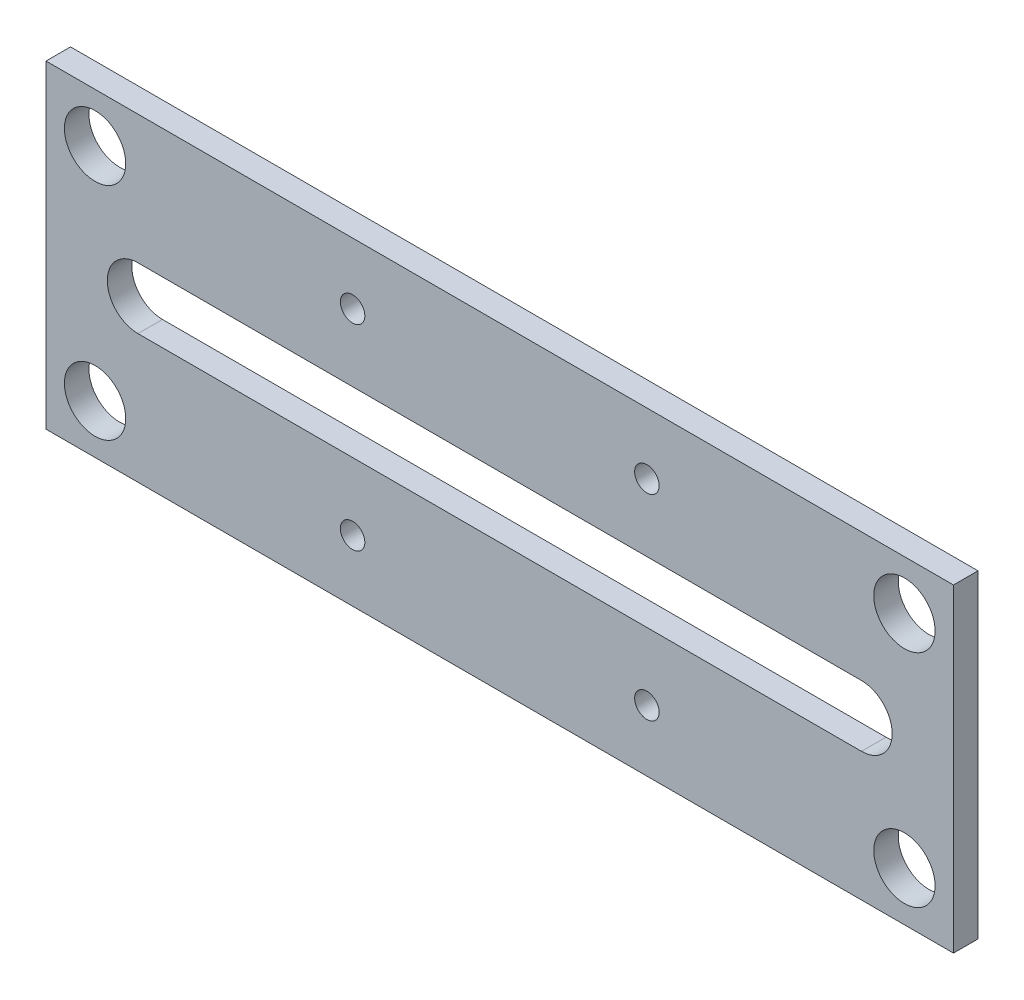
SolidWorks part; units mm, degrees
ref_plane "Front Plane" through (0, 0, 0) normal (0, 0, 1) x (1, 0, 0)
ref_plane "Top Plane" through (0, 0, 0) normal (0, 1, 0) x (1, 0, 0)
ref_plane "Right Plane" through (0, 0, 0) normal (1, 0, 0) x (0, 0, -1)
ref_plane "Plane1" through (0, 0, 0) normal (0, 0, -1) x (-1, 0, 0)
sketch "Sketch1" plane through (0, 0, 0) normal (0, 0, -1) x (-1, 0, 0)
  line L0 (-185, 0) -> (-185, 6.1768) construction
  line L1 (0, 0) -> (0, 130)
  line L3 (0, 130) -> (-370, 130)
  line L5 (-370, 130) -> (-370, 0)
  line L7 (-370, 0) -> (0, 0)
  line L8 (-37.5, 52.5) -> (-332.5, 52.5)
  line L9 (-332.5, 77.5) -> (-37.5, 77.5)
  line L10 (0, 65) -> (-33.5774, 65) construction
  line L11 (-370, 65) -> (-332.5, 65) construction
  line L12 (-185, 130) -> (-185, 77.5) construction
  circle A6 centre (-350, 20) radius 12.5
  circle A7 centre (-20, 110) radius 12.5
  arc A8 (-37.5, 77.5) -> (-37.5, 52.5) centre (-37.5, 65) cw
  arc A9 (-332.5, 52.5) -> (-332.5, 77.5) centre (-332.5, 65) cw
  circle A10 centre (-350, 110) radius 12.5
  circle A11 centre (-20, 20) radius 12.5
  dimension "D1" = 25
  dimension "D2" = 25
  dimension "D3" = 330
  dimension "D4" = 90
  dimension "D5" = 130
  dimension "D6" = 370
  dimension "D7" = 295
extrude "Boss-Extrude1" add sketch "Sketch1" against normal blind 10
hole_wizard "M8 Clearance Hole1" positions "Sketch5" profile "Sketch6" hole size "M8" standard "GB" end condition through all
sketch "Sketch5" plane through (0, 0, 0) normal (0, 0, -1) x (-1, 0, 0)
  line L0 (-332.5, 65) -> (-37.5, 65) construction
  line L2 (-185, 65) -> (-185, 0) construction
  line L4 (0, 130) -> (-370, 130) construction
  line L5 (-370, 0) -> (0, 0) construction
  point P0 (-245, 25)
  point P2 (-125, 25)
  point P13 (-125, 105)
  point P14 (-245, 105)
  dimension "D1" = 120
  dimension "D2" = 25
sketch "Sketch6" plane through (245, 25, 0) normal (1, 0, 0) x (0, 1, 0)
  line L0 (0, 0) -> (0, 10)
  line L1 (0, 10) -> (5, 10)
  line L2 (5, 10) -> (5, 0)
  line L5 (5, 0) -> (0, 0)
  line L11 (0, -6.35) -> (0, 107.95) construction
  dimension "通孔孔直径" = 10
  dimension "通孔孔深度" = 10
